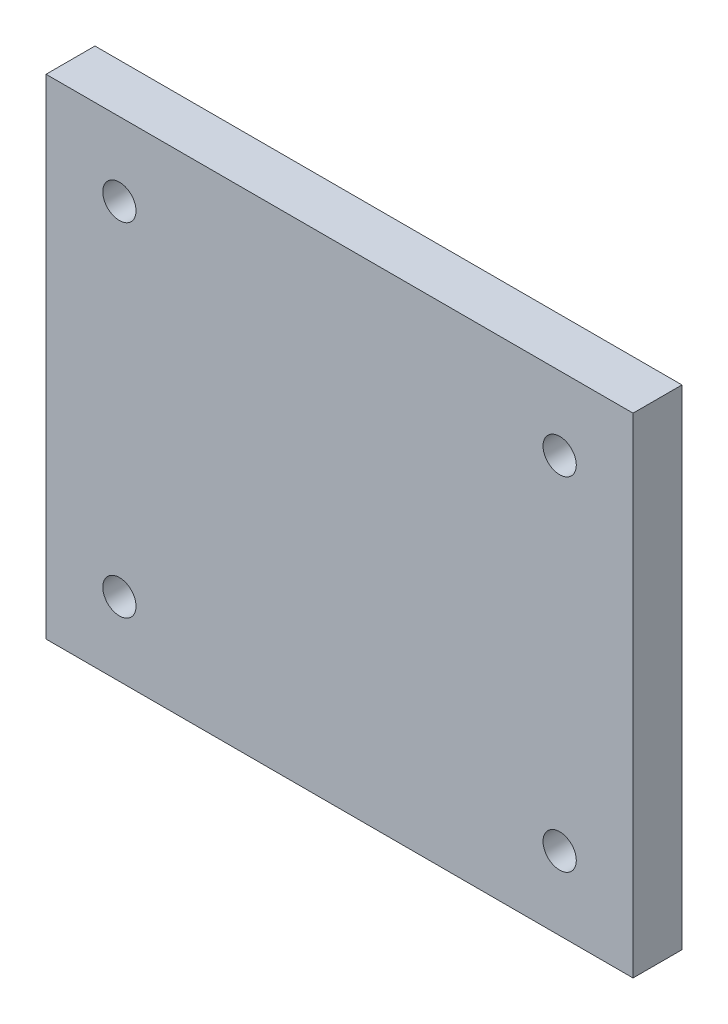
SolidWorks part; units mm, degrees
material "1023 碳钢板 (SS)"
ref_plane "Front Plane" through (0, 0, 0) normal (0, 0, 1) x (1, 0, 0)
ref_plane "Top Plane" through (0, 0, 0) normal (0, 1, 0) x (1, 0, 0)
ref_plane "Right Plane" through (0, 0, 0) normal (1, 0, 0) x (0, 0, -1)
sketch "Sketch1" plane through (0, 0, 0) normal (0, 0, 1) x (1, 0, 0)
  line L1 (60, 50) -> (-60, 50)
  line L2 (60, 50) -> (60, -50)
  line L3 (60, -50) -> (-60, -50)
  line L4 (-60, 50) -> (-60, -50)
  line L5 (60, 50) -> (-60, -50) construction
  line L6 (60, -50) -> (-60, 50) construction
  point P0 (0, 0)
  dimension "D1" = 120
  dimension "D2" = 100
extrude "Boss-Extrude1" add sketch "Sketch1" along normal blind 10
sketch "Sketch2" plane through (0, 0, 10) normal (0, 0, 1) x (1, 0, 0)
  line L1 (45, 35) -> (-45, 35) construction
  line L2 (45, 35) -> (45, -35) construction
  line L3 (45, -35) -> (-45, -35) construction
  line L4 (-45, 35) -> (-45, -35) construction
  line L5 (45, 35) -> (-45, -35) construction
  line L6 (45, -35) -> (-45, 35) construction
  circle A0 centre (-45, 35) radius 3
  circle A1 centre (45, 35) radius 3
  circle A2 centre (45, -35) radius 3
  circle A3 centre (-45, -35) radius 3
  point P0 (0, 0)
  dimension "D3" = 6
  dimension "D1" = 90
  dimension "D2" = 70
hole_wizard "M8 Tapped Hole1" positions "Sketch5" profile "Sketch6" tap size "M8" standard "ISO"
sketch "Sketch5" plane through (0, 0, 10) normal (0, 0, 1) x (1, 0, 0)
  point P0 (45, -35)
  point P3 (-45, -35)
  point P6 (-45, 35)
  point P9 (45, 35)
sketch "Sketch6" plane through (45, -35, 10) normal (1, 0, 0) x (0, -1, 0)
  line L0 (0, 0) -> (0, 21.7929)
  line L1 (0, 21.7929) -> (3.4, 19.75)
  line L2 (3.4, 19.75) -> (3.4, 0)
  line L5 (3.4, 0) -> (0, 0)
  line L10 (0, 21.7929) -> (-3.4, 19.75) construction
  line L11 (0, -6.35) -> (0, 107.95) construction
  dimension "螺纹孔钻头直径" = 6.8
  dimension "螺纹孔钻头深度" = 19.75
  dimension "导头角度" = 118
cosmetic thread "Hole Thread Line 1" parameters "D1"=16, "D2"=8
cosmetic thread "Hole Thread Line 2" parameters "D1"=16, "D2"=8
cosmetic thread "Hole Thread Line 3" parameters "D1"=16, "D2"=8
cosmetic thread "Hole Thread Line 4" parameters "D1"=16, "D2"=8
